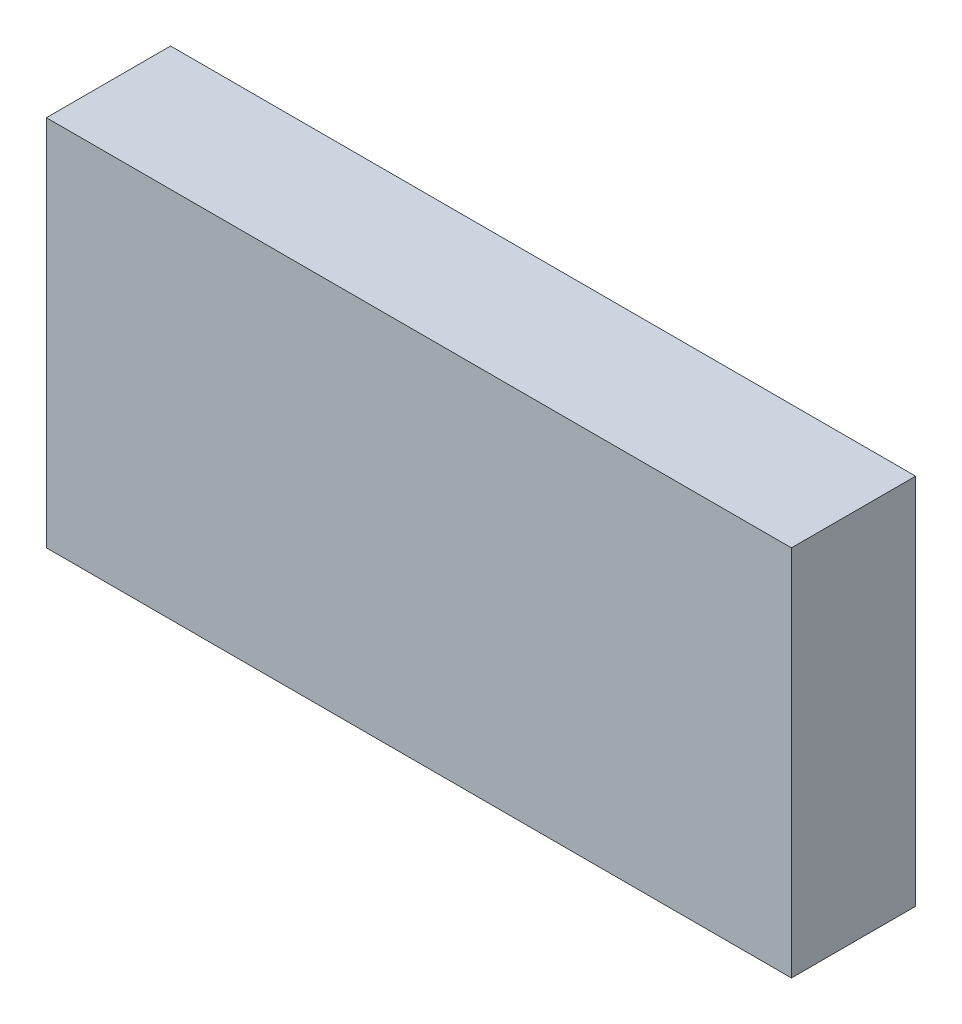
SolidWorks part; units mm, degrees
material "Q235B"
ref_plane "Front Plane" through (0, 0, 0) normal (0, 0, 1) x (1, 0, 0)
ref_plane "Top Plane" through (0, 0, 0) normal (0, 1, 0) x (1, 0, 0)
ref_plane "Right Plane" through (0, 0, 0) normal (1, 0, 0) x (0, 0, -1)
sketch "Sketch1" plane through (0, 0, 0) normal (0, 0, 1) x (1, 0, 0)
  line L1 (0, 0) -> (120, 0)
  line L2 (0, 0) -> (0, 60)
  line L3 (0, 60) -> (120, 60)
  line L4 (120, 0) -> (120, 60)
  dimension "D1" = 120
  dimension "D2" = 60
extrude "Boss-Extrude1" add sketch "Sketch1" along normal blind 20
